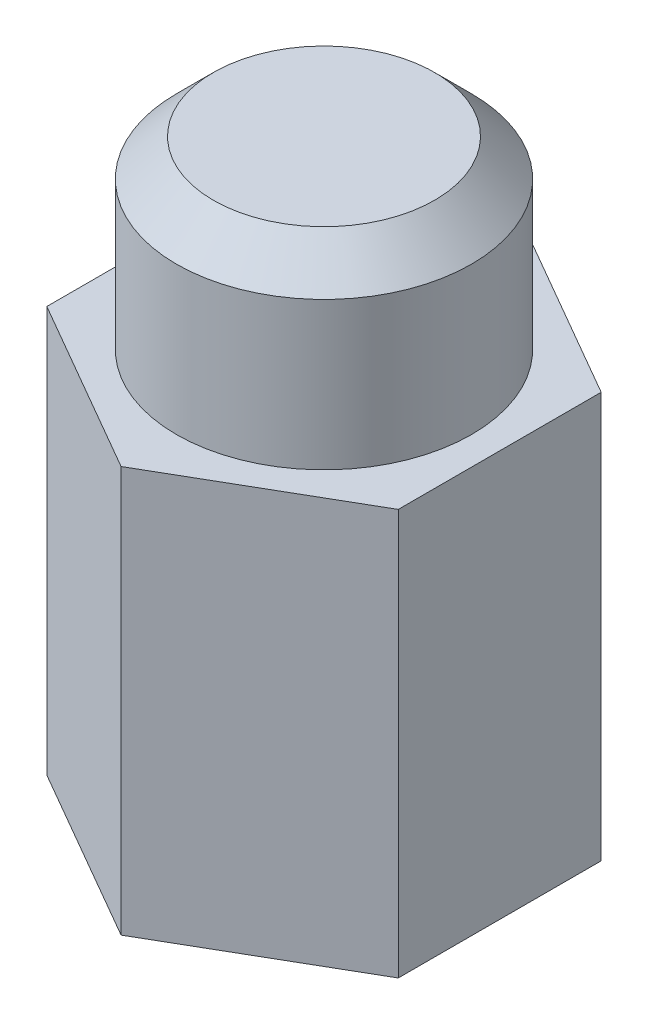
from build123d import *

# Parameters (mm, degrees)
BOSS_EXTRUDE1_DEPTH       = 5.5
SKETCH3_R                 = 4
BOSS_EXTRUDE2_DEPTH       = 5
CHAMFER1_SIZE             = 1
M6X1_0_TAPPED_HOLE1_D     = 5
M6X1_0_TAPPED_HOLE1_DEPTH = 8
M6X1_0_TAPPED_HOLE1_TIP   = 1.502151548


with BuildPart() as part:
    # Sketch1 → Boss-Extrude1 (new, symmetric)
    with BuildSketch(Plane(origin=(0, 0, 0), x_dir=(1, 0, 0), z_dir=(0, 1, 0))):
        Polygon((0, 5.5), (-4.763139721, 2.75), (-4.763139721, -2.75), (0, -5.5), (4.763139721, -2.75), (4.763139721, 2.75), align=None)
    extrude(amount=BOSS_EXTRUDE1_DEPTH, both=True)

    # Sketch3 → Boss-Extrude2 (add)
    with BuildSketch(Plane(origin=(0, 5.5, 0), x_dir=(1, 0, 0), z_dir=(0, 1, 0))):
        with Locations(Location((0, 0, 0), (0, 0, 270))):
            Circle(SKETCH3_R)
    extrude(amount=BOSS_EXTRUDE2_DEPTH)

    # Chamfer1
    chamfer1_edges = [part.edges().sort_by_distance(p)[0] for p in [
        (0, 10.5, -4),
    ]]
    chamfer(chamfer1_edges, length=CHAMFER1_SIZE)

    # M6x1.0 Tapped Hole1
    with Locations(Plane(origin=(0, -5.5, 0), x_dir=(-1, 0, 0), z_dir=(0, -1, 0))):
        with Locations((-0.001364709, 0)):
            Hole(M6X1_0_TAPPED_HOLE1_D / 2, depth=M6X1_0_TAPPED_HOLE1_DEPTH)
            with Locations((0, 0, -(M6X1_0_TAPPED_HOLE1_DEPTH + M6X1_0_TAPPED_HOLE1_TIP / 2))):  # 118° drill point
                Cone(0, M6X1_0_TAPPED_HOLE1_D / 2, M6X1_0_TAPPED_HOLE1_TIP, mode=Mode.SUBTRACT)


solid = part.part
